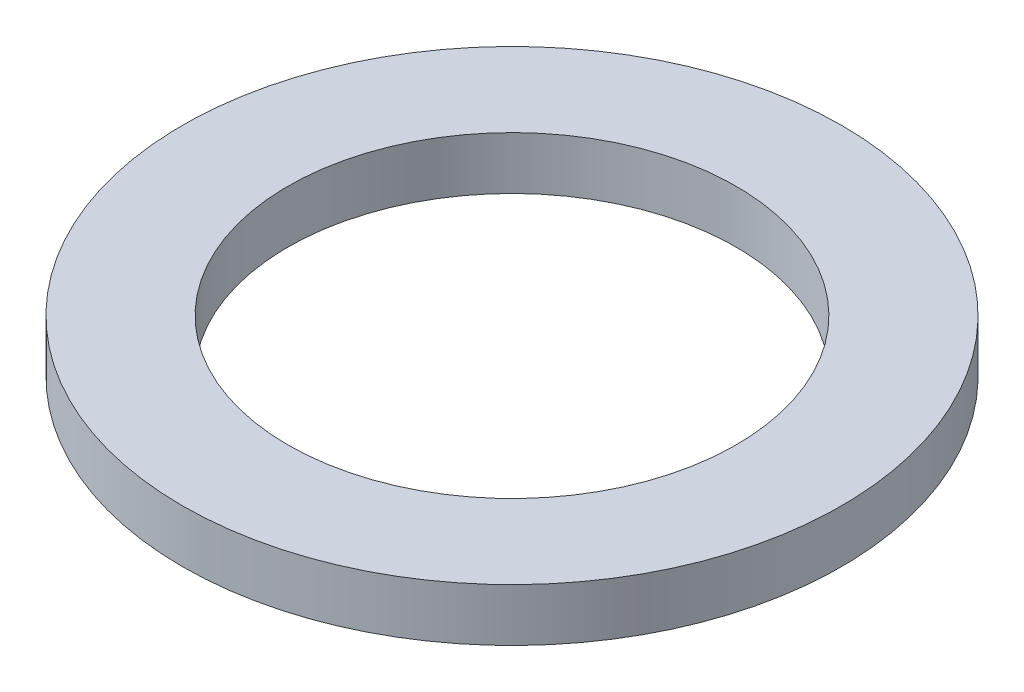
SolidWorks part; units mm, degrees
ref_plane "Front Plane" through (0, 0, 0) normal (0, 0, 1) x (1, 0, 0)
ref_plane "Top Plane" through (0, 0, 0) normal (0, 1, 0) x (1, 0, 0)
ref_plane "Right Plane" through (0, 0, 0) normal (1, 0, 0) x (0, 0, -1)
other "Configuration Table"
sketch "Sketch1" plane through (0, 0, 0) normal (0, 1, 0) x (1, 0, 0)
  circle A0 centre (0, 0) radius 12.5
  circle A1 centre (0, 0) radius 8.5
  dimension "D1" = 25
  dimension "D2" = 17
extrude "Boss-Extrude1" add sketch "Sketch1" along normal blind 2
